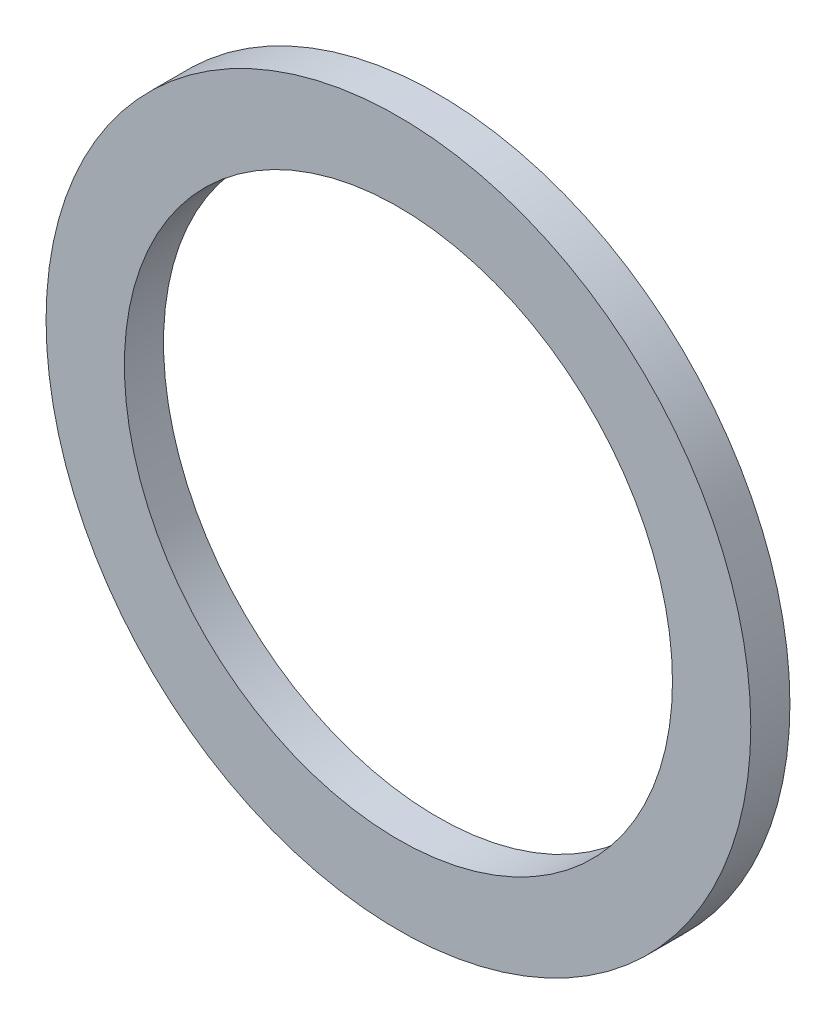
SolidWorks part; units mm, degrees
ref_plane "前视基准面" through (0, 0, 0) normal (0, 0, 1) x (1, 0, 0)
ref_plane "上视基准面" through (0, 0, 0) normal (0, 1, 0) x (1, 0, 0)
ref_plane "右视基准面" through (0, 0, 0) normal (1, 0, 0) x (0, 0, -1)
sketch "草图1" plane through (0, 0, 0) normal (0, 0, 1) x (1, 0, 0)
  circle A0 centre (0, 0) radius 22.5
  circle A1 centre (0, 0) radius 17.5
  dimension "D1" = 35
  dimension "D2" = 45
extrude "凸台-拉伸1" add sketch "草图1" along normal blind 2.5
